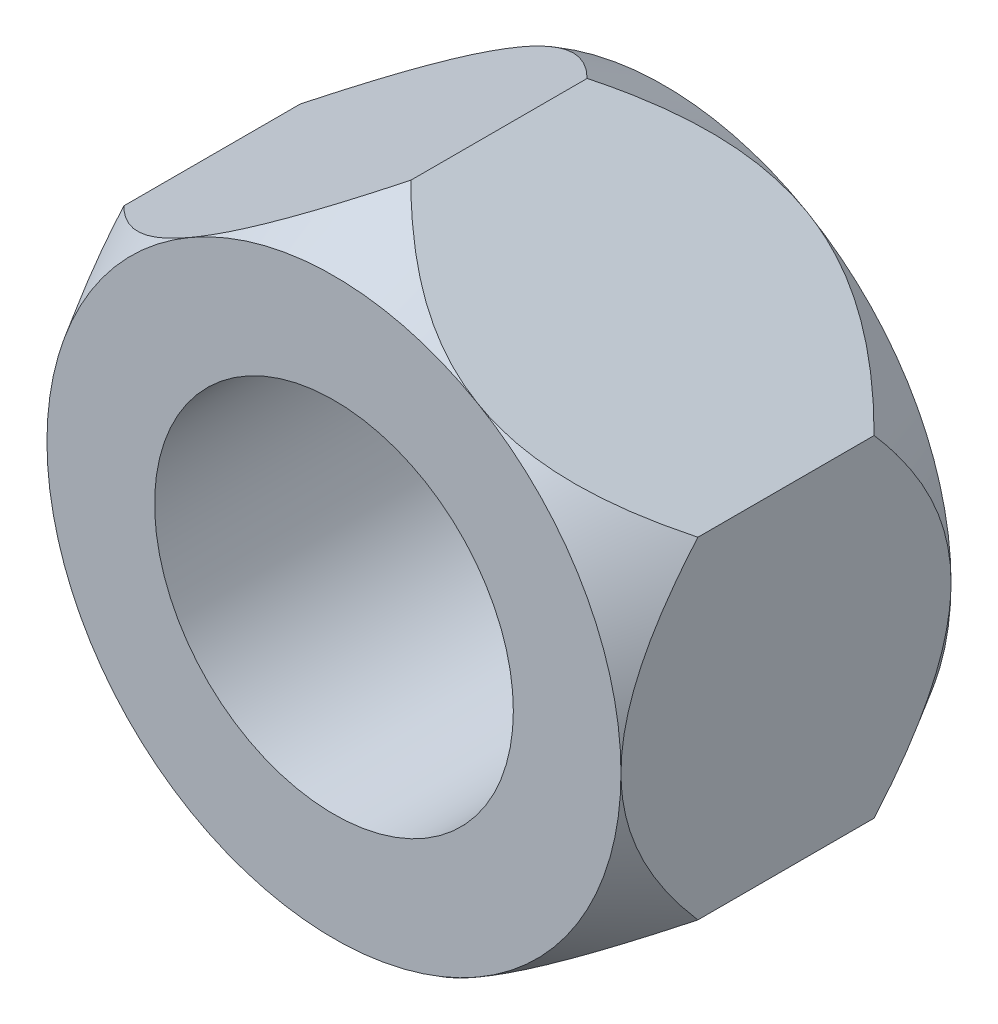
from build123d import *

# Parameters (mm, degrees)
BOSS_EXTRUDE1_DEPTH     = 11.5
SKETCH2_OUTSIDE_W       = 75.842
SKETCH2_OUTSIDE_H       = 82.03
SKETCH2_OUTSIDE_R       = 20
CUT_EXTRUDE1_DEPTH      = 18
CUT_EXTRUDE1_DRAFT      = -30
MIRROR1_COPY_1_SKETCH_W = 75.842
MIRROR1_COPY_1_SKETCH_H = 82.03
MIRROR1_COPY_1_SKETCH_R = 20
MIRROR1_COPY_1_DEPTH    = 18
MIRROR1_COPY_1_DRAFT    = -30
SKETCH3_R               = 12.5
CUT_EXTRUDE2_DEPTH      = 18
SKETCH4_R               = 6
CUT_EXTRUDE3_DEPTH      = 18


with BuildPart() as part:
    # Sketch1 → Boss-Extrude1 (new, symmetric)
    with BuildSketch(Plane.XY):
        Polygon((0, 23.094010768), (-20, 11.547005384), (-20, -11.547005384), (0, -23.094010768), (20, -11.547005384), (20, 11.547005384), align=None)
    extrude(amount=BOSS_EXTRUDE1_DEPTH, both=True)


with BuildPart() as cut_extrude1_tool:
    # Sketch2 outside → Cut-Extrude1 (with draft: the straight prism first)
    with BuildSketch(Plane.XY.offset(11.5)):
        Rectangle(SKETCH2_OUTSIDE_W, SKETCH2_OUTSIDE_H)
        Circle(SKETCH2_OUTSIDE_R, mode=Mode.SUBTRACT)
    extrude(amount=-CUT_EXTRUDE1_DEPTH)
    # Cut-Extrude1: the draft: its side faces are tilted about the plane it starts from
    cut_extrude1_sides = [cut_extrude1_tool.faces().sort_by_distance(p)[0] for p in [
        (0, -41.015, 2.5),
        (37.921, 0, 2.5),
        (0, 41.015, 2.5),
        (-37.921, 0, 2.5),
        (-20, 0, 2.5),
    ]]
    draft(cut_extrude1_sides, Plane.XY.offset(11.5), CUT_EXTRUDE1_DRAFT)


with BuildPart() as part_1:
    add(part.part)

    # Cut-Extrude1: cut by cut_extrude1_tool
    add(cut_extrude1_tool.part, mode=Mode.SUBTRACT)


with BuildPart() as mirror1_copy_1_tool:
    # Mirror1 copy 1 sketch → Mirror1 copy 1 (with draft: the straight prism first)
    with BuildSketch(Plane(origin=(0, 0, -11.5), x_dir=(1, 0, 0), z_dir=(0, 0, -1))):
        Rectangle(MIRROR1_COPY_1_SKETCH_W, MIRROR1_COPY_1_SKETCH_H)
        Circle(MIRROR1_COPY_1_SKETCH_R, mode=Mode.SUBTRACT)
    extrude(amount=-MIRROR1_COPY_1_DEPTH)
    # Mirror1 copy 1: the draft: its side faces are tilted about the plane it starts from
    mirror1_copy_1_sides = [mirror1_copy_1_tool.faces().sort_by_distance(p)[0] for p in [
        (0, -41.015, -2.5),
        (37.921, 0, -2.5),
        (0, 41.015, -2.5),
        (-37.921, 0, -2.5),
        (-20, 0, -2.5),
    ]]
    draft(mirror1_copy_1_sides, Plane(origin=(0, 0, -11.5), x_dir=(1, 0, 0), z_dir=(0, 0, -1)), MIRROR1_COPY_1_DRAFT)


with BuildPart() as part_2:
    add(part_1.part)

    # Mirror1 copy 1: cut by mirror1_copy_1_tool
    add(mirror1_copy_1_tool.part, mode=Mode.SUBTRACT)

    # Sketch3 → Cut-Extrude2 (cut)
    with BuildSketch(Plane.XY.offset(11.5)):
        Circle(SKETCH3_R)
    extrude(amount=-CUT_EXTRUDE2_DEPTH, mode=Mode.SUBTRACT)

    # Sketch4 → Cut-Extrude3 (cut)
    with BuildSketch(Plane.XY.offset(-6.5)):
        Circle(SKETCH4_R)
    extrude(amount=-CUT_EXTRUDE3_DEPTH, mode=Mode.SUBTRACT)


solid = part_2.part
